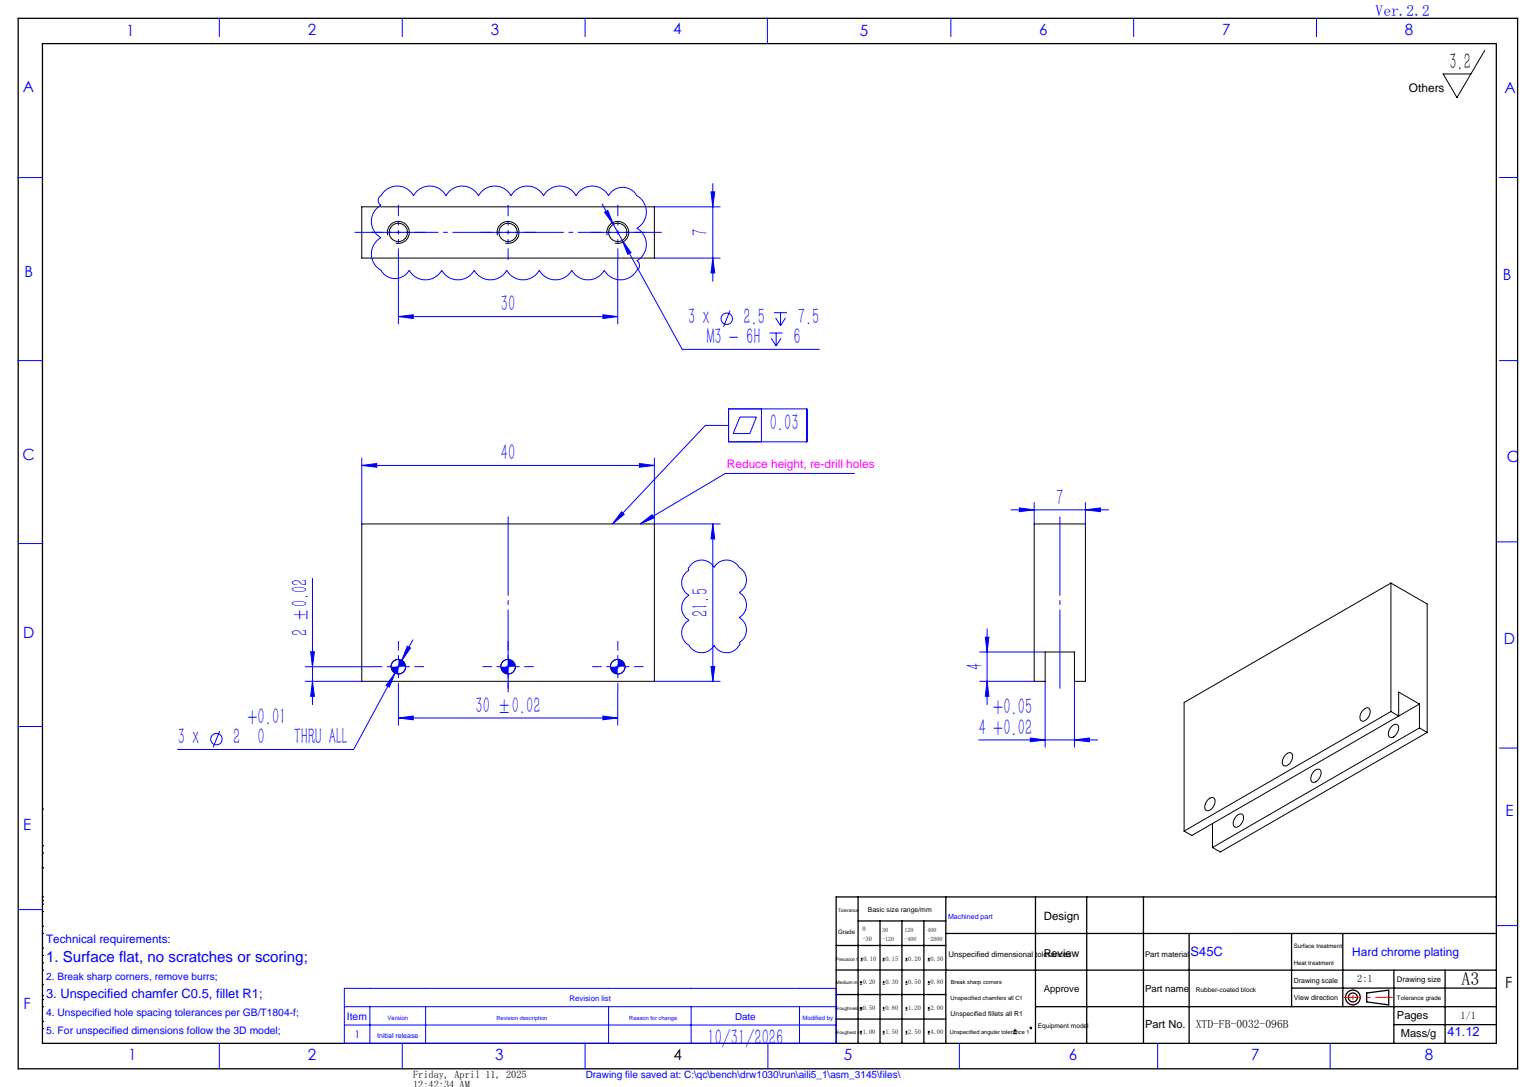
from build123d import *

# Parameters (mm, degrees)
SKETCH_1_W             = 40
SKETCH_1_H             = 7
EXTRUDE_1_DEPTH        = 21.5
HOLE_WIZARD_M3_1_D     = 2.5
HOLE_WIZARD_M3_1_DEPTH = 7.5
HOLE_WIZARD_M3_1_TIP   = 0.751075774
SKETCH_4_W             = 4
SKETCH_4_H             = 4
CUT_EXTRUDE_1_DEPTH    = 46.546679352
MM_1_D                 = 2


with BuildPart() as part:
    # 草图1 → 凸台-拉伸1 (new body)
    with BuildSketch(Plane.XY):
        Rectangle(SKETCH_1_W, SKETCH_1_H)
    extrude(amount=EXTRUDE_1_DEPTH)

    # M3 螺纹孔1
    with Locations(Plane.XY.offset(21.5)):
        with Locations((-15, 0), (0, 0), (15, 0)):
            Hole(HOLE_WIZARD_M3_1_D / 2, depth=HOLE_WIZARD_M3_1_DEPTH)
            with Locations((0, 0, -(HOLE_WIZARD_M3_1_DEPTH + HOLE_WIZARD_M3_1_TIP / 2))):  # 118° drill point
                Cone(0, HOLE_WIZARD_M3_1_D / 2, HOLE_WIZARD_M3_1_TIP, mode=Mode.SUBTRACT)

    # 草图4 → 切除-拉伸1 (cut, through all)
    with BuildSketch(Plane(origin=(20, 0, 0), x_dir=(0, 0, -1), z_dir=(1, 0, 0))):
        with Locations((-2, 0)):
            Rectangle(SKETCH_4_W, SKETCH_4_H)
    extrude(amount=-CUT_EXTRUDE_1_DEPTH, mode=Mode.SUBTRACT)

    # 大小mm 暗销孔1 (through all)
    with Locations(Plane(origin=(0, 3.5, 0), x_dir=(1, 0, 0), z_dir=(0, 1, 0))):
        with Locations((-15, -2), (0, -2), (15, -2)):
            Hole(MM_1_D / 2)


solid = part.part
